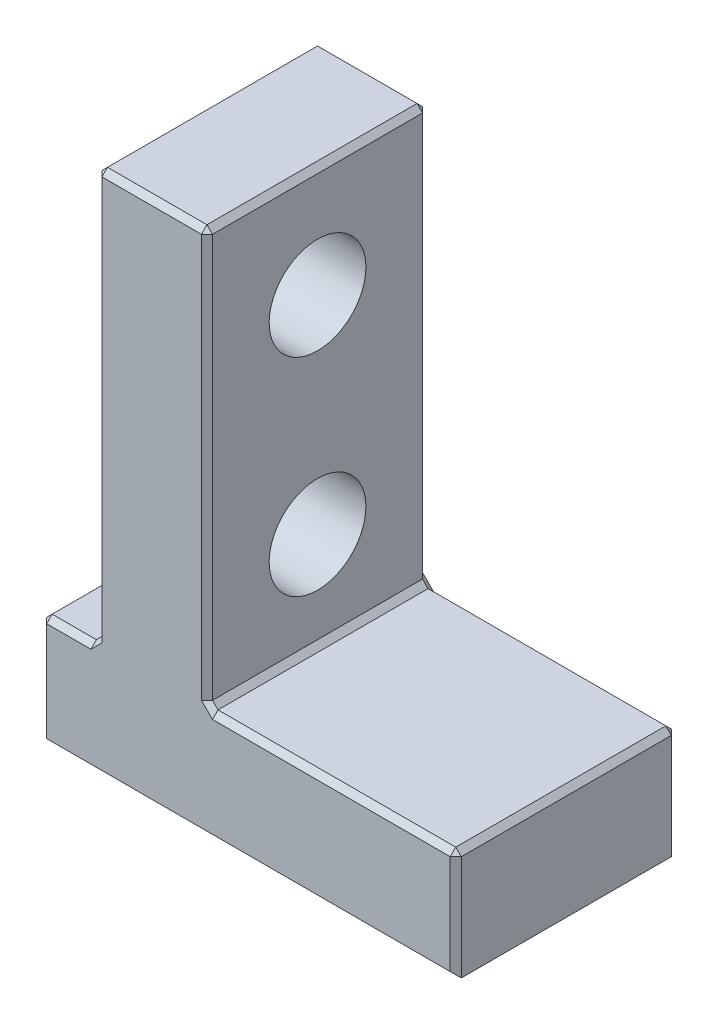
from build123d import *

# Parameters (mm, degrees)
BOSS_EXTRUDE1_DEPTH            = 8
CHAMFER1_SIZE                  = 0.2
CUT_EXTRUDE1_REACH             = 23.401
SKETCH4_R                      = 1.75
CUT_EXTRUDE1_DIRECTION_2_DEPTH = 22.400934559


with BuildPart() as part:
    # Sketch2 → Boss-Extrude1 (new body)
    with BuildSketch(Plane.XY):
        Polygon((-10.793974552, 0), (-8.793974552, 0), (-8.793974552, 15), (-4.793974552, 15), (-4.793974552, 0), (4.206025448, 0), (4.206025448, -4), (-10.793974552, -4), align=None)
    extrude(amount=BOSS_EXTRUDE1_DEPTH)

    # Chamfer1
    chamfer1_edges = [part.edges().sort_by_distance(p)[0] for p in [
        (-0.293974552, 0, 0),
        (4.206025448, -2, 0),
        (-3.293974552, -4, 0),
        (-10.793974552, -2, 0),
        (4.206025448, -2, 8),
        (-10.793974552, 0, 4),
        (-8.793974552, 0, 4),
        (-8.793974552, 15, 4),
        (-4.793974552, 15, 4),
        (-4.793974552, 0, 4),
        (4.206025448, 0, 4),
        (-10.793974552, -4, 4),
        (-0.293974552, 0, 8),
        (-4.793974552, 7.5, 8),
        (-6.793974552, 15, 8),
        (-8.793974552, 7.5, 8),
        (-9.793974552, 0, 8),
        (-10.793974552, -2, 8),
        (-9.793974552, 0, 0),
        (-3.293974552, -4, 8),
        (-8.793974552, 7.5, 0),
        (-6.793974552, 15, 0),
        (-4.793974552, 7.5, 0),
    ]]
    chamfer(chamfer1_edges, length=CHAMFER1_SIZE)

    # Sketch4 → Cut-Extrude1 (cut, up to next)
    with BuildSketch(Plane.ZY.offset(8.793974552), mode=Mode.PRIVATE) as cut_extrude1_sk1:
        with Locations(Location((4, 11, 0), (0, 0, 180))):
            Circle(SKETCH4_R)
    cut_extrude1_tool1 = extrude(cut_extrude1_sk1.sketch, amount=-CUT_EXTRUDE1_REACH, mode=Mode.PRIVATE) & part.part
    # Sketch4 → Cut-Extrude1 (cut, up to next)
    with BuildSketch(Plane.ZY.offset(8.793974552), mode=Mode.PRIVATE) as cut_extrude1_sk2:
        with Locations(Location((4, 3.5, 0), (0, 0, 180))):
            Circle(SKETCH4_R)
    cut_extrude1_tool2 = extrude(cut_extrude1_sk2.sketch, amount=-CUT_EXTRUDE1_REACH, mode=Mode.PRIVATE) & part.part
    add(cut_extrude1_tool1.solids().sort_by_distance((-8.793975, 11, 4))[0], mode=Mode.SUBTRACT)
    add(cut_extrude1_tool2.solids().sort_by_distance((-8.793975, 3.5, 4))[0], mode=Mode.SUBTRACT)

    # Sketch4 → Cut-Extrude1 direction 2 (cut)
    with BuildSketch(Plane.ZY.offset(8.793974552)):
        with Locations(Location((4, 11, 0), (0, 0, 180))):
            Circle(SKETCH4_R)
        with Locations(Location((4, 3.5, 0), (0, 0, 180))):
            Circle(SKETCH4_R)
    extrude(amount=CUT_EXTRUDE1_DIRECTION_2_DEPTH, mode=Mode.SUBTRACT)


solid = part.part
